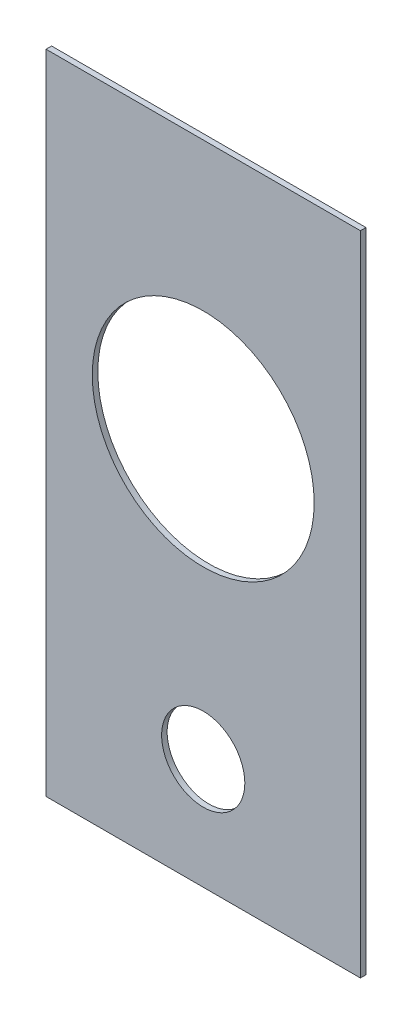
SolidWorks part; units mm, degrees
ref_plane "Front Plane" through (0, 0, 0) normal (0, 0, 1) x (1, 0, 0)
ref_plane "Top Plane" through (0, 0, 0) normal (0, 1, 0) x (1, 0, 0)
ref_plane "Right Plane" through (0, 0, 0) normal (1, 0, 0) x (0, 0, -1)
sketch "Sketch1" plane through (0, 0, 0) normal (0, 0, 1) x (1, 0, 0)
  line L1 (0, 0) -> (170, 0)
  line L2 (0, 0) -> (0, 350)
  line L3 (0, 350) -> (170, 350)
  line L4 (170, 0) -> (170, 350)
  circle A0 centre (85, 210) radius 60
  circle A1 centre (85, 60) radius 22.5
  dimension "D3" = 140
  dimension "D5" = 120
  dimension "D6" = 45
  dimension "D1" = 170
  dimension "D2" = 350
  dimension "D4" = 150
  dimension "D7" = 85
  dimension "D8" = 85
extrude "Boss-Extrude1" add sketch "Sketch1" along normal blind 3
